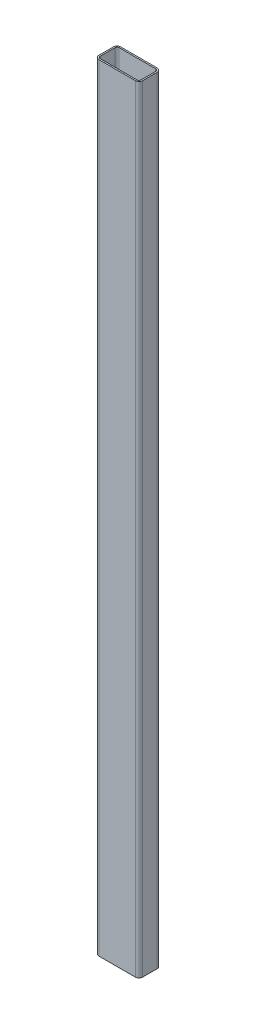
from build123d import *

# Parameters (mm, degrees)
EXTRUDE_THIN1_DEPTH = 1062


with BuildPart() as part:
    # Sketch1 → Extrude-Thin1 (new, symmetric)
    with BuildSketch(Plane(origin=(0, 0, 0), x_dir=(1, 0, 0), z_dir=(0, 1, 0))):
        with BuildLine():
            Line((-50, 30), (50, 30))
            ThreePointArc((50, 30), (57.071067812, 27.071067812), (60, 20))
            Line((60, 20), (60, -20))
            ThreePointArc((60, -20), (57.071067812, -27.071067812), (50, -30))
            Line((50, -30), (-50, -30))
            ThreePointArc((-50, -30), (-57.071067812, -27.071067812), (-60, -20))
            Line((-60, -20), (-60, 20))
            ThreePointArc((-60, 20), (-57.071067812, 27.071067812), (-50, 30))
        make_face()
        with BuildLine():
            Line((-50, 26), (50, 26))
            ThreePointArc((50, 26), (54.242640687, 24.242640687), (56, 20))
            Line((56, 20), (56, -20))
            ThreePointArc((56, -20), (54.242640687, -24.242640687), (50, -26))
            Line((50, -26), (-50, -26))
            ThreePointArc((-50, -26), (-54.242640687, -24.242640687), (-56, -20))
            Line((-56, -20), (-56, 20))
            ThreePointArc((-56, 20), (-54.242640687, 24.242640687), (-50, 26))
        make_face(mode=Mode.SUBTRACT)
    extrude(amount=EXTRUDE_THIN1_DEPTH, both=True)


solid = part.part
